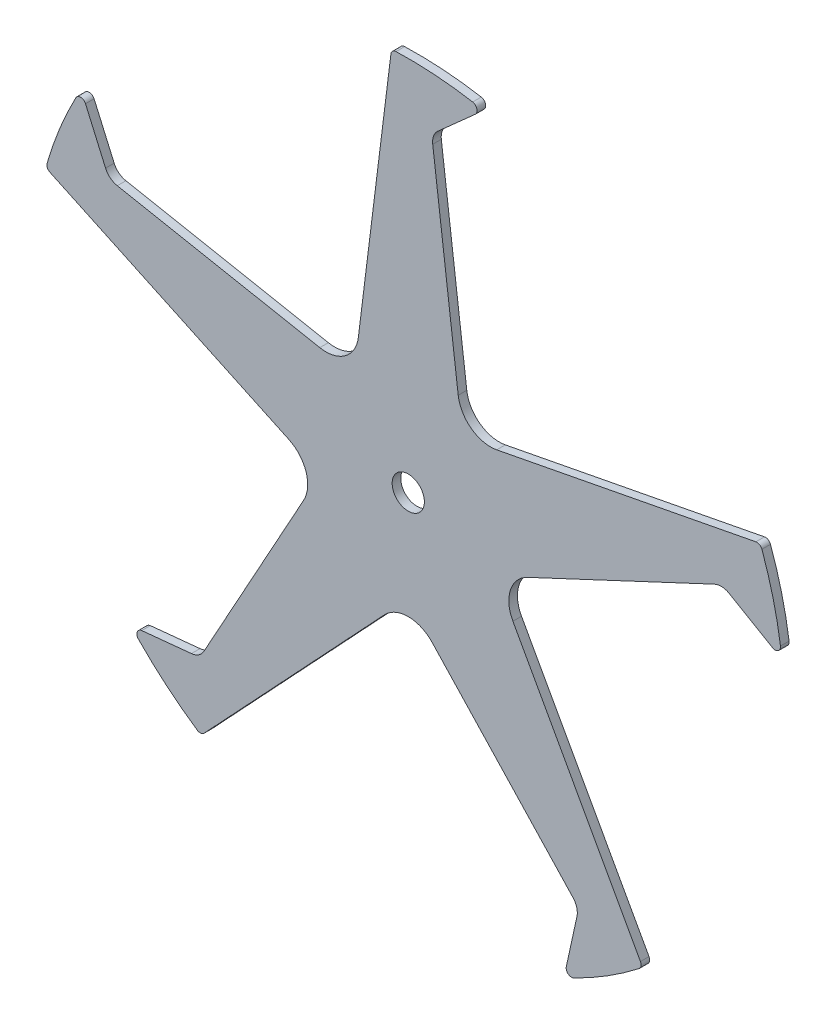
SolidWorks part; units mm, degrees
ref_plane "Front Plane" through (0, 0, 0) normal (0, 0, 1) x (1, 0, 0)
ref_plane "Top Plane" through (0, 0, 0) normal (0, 1, 0) x (1, 0, 0)
ref_plane "Right Plane" through (0, 0, 0) normal (1, 0, 0) x (0, 0, -1)
sketch "Sketch1" plane through (0, 0, 0) normal (0, 0, 1) x (1, 0, 0)
  line L0 (-46.4905, 101.7221) -> (-16.1451, 345.4365)
  line L1 (46.4905, 101.7221) -> (22.7757, 292.1841)
  line L2 (0, -284.2155) -> (0, 291.5871) construction
  line L3 (21.8025, 300) -> (-21.8025, 300) construction
  line L4 (82.3771, 75.649) -> (323.5405, 122.1007)
  line L5 (111.1098, -12.7813) -> (284.9216, 68.6289)
  line L6 (298.854, 67.9948) -> (339.0018, 44.5257)
  line L7 (292.0543, 71.9697) -> (278.5796, 113.4405) construction
  line L8 (97.4024, -54.9684) -> (216.1041, -269.9741)
  line L9 (22.1791, -109.6213) -> (153.3156, -249.7691)
  line L10 (157.0179, -263.2155) -> (147.1038, -308.6507)
  line L11 (158.697, -255.5203) -> (193.9742, -229.8899) construction
  line L12 (27.6841, 305.2386) -> (62.4109, 336.1691)
  line L13 (-22.1791, -109.6213) -> (-189.9808, -288.9539)
  line L14 (-97.4024, -54.9684) -> (-190.1674, -222.9947)
  line L15 (-201.8116, -230.6709) -> (-248.0867, -235.2823)
  line L16 (-193.9742, -229.8899) -> (-158.697, -255.5203) construction
  line L17 (-111.1098, -12.7813) -> (-333.5187, 91.3908)
  line L18 (-82.3771, 75.649) -> (-270.8455, 111.9508)
  line L19 (-281.7443, 120.6531) -> (-300.4298, 163.2382)
  line L20 (-278.5796, 113.4405) -> (-292.0543, 71.9697) construction
  arc A0 (59.9416, 344.8289) -> (-11.3455, 349.8161) centre (0, 0) ccw
  circle A1 centre (0, 0) radius 100 construction
  arc A2 (27.6841, 305.2386) -> (22.7757, 292.1841) centre (37.6608, 294.0374) ccw
  circle A3 centre (0, 0) radius 350 construction
  arc A4 (59.9416, 344.8289) -> (62.4109, 336.1691) centre (59.0853, 339.9028) cw
  arc A5 (-11.3455, 349.8161) -> (-16.1451, 345.4365) centre (-11.1834, 344.8187) ccw
  arc A6 (346.4748, 49.5501) -> (329.1889, 118.8893) centre (0, 0) ccw
  arc A7 (298.854, 67.9948) -> (284.9216, 68.6289) centre (291.284, 55.0451) ccw
  arc A8 (346.4748, 49.5501) -> (339.0018, 44.5257) centre (341.5252, 48.8423) cw
  arc A9 (329.1889, 118.8893) -> (323.5405, 122.1007) centre (324.4862, 117.1909) ccw
  arc A10 (154.1916, -314.2053) -> (214.7954, -276.3384) centre (0, 0) ccw
  arc A11 (157.0179, -263.2155) -> (153.3156, -249.7691) centre (142.3627, -260.0177) ccw
  arc A12 (154.1916, -314.2053) -> (147.1038, -308.6507) centre (151.9888, -309.7166) cw
  arc A13 (214.7954, -276.3384) -> (216.1041, -269.9741) centre (211.7269, -272.3907) ccw
  arc A14 (-251.1792, -243.7397) -> (-196.438, -289.6759) centre (0, 0) ccw
  arc A15 (-201.8116, -230.6709) -> (-190.1674, -222.9947) centre (-203.2991, -215.7448) ccw
  arc A16 (-251.1792, -243.7397) -> (-248.0867, -235.2823) centre (-247.5909, -240.2577) cw
  arc A17 (-196.438, -289.6759) -> (-189.9808, -288.9539) centre (-193.6318, -285.5376) ccw
  arc A18 (-309.4288, 163.5659) -> (-336.2008, 97.3089) centre (0, 0) ccw
  arc A19 (-281.7443, 120.6531) -> (-270.8455, 111.9508) centre (-268.0084, 126.6801) ccw
  arc A20 (-309.4288, 163.5659) -> (-300.4298, 163.2382) centre (-305.0084, 161.2292) cw
  arc A21 (-336.2008, 97.3089) -> (-333.5187, 91.3908) centre (-331.3979, 95.9188) ccw
  arc A22 (82.3771, 75.649) -> (46.4905, 101.7221) centre (76.6321, 105.4751) cw
  arc A23 (97.4024, -54.9684) -> (111.1098, -12.7813) centre (123.9934, -40.2879) cw
  arc A24 (-22.1791, -109.6213) -> (22.1791, -109.6213) centre (0, -130.3744) cw
  arc A25 (-111.1098, -12.7813) -> (-97.4024, -54.9684) centre (-123.9934, -40.2879) cw
  arc A26 (-46.4905, 101.7221) -> (-82.3771, 75.649) centre (-76.6321, 105.4751) cw
  circle A27 centre (0, 0) radius 15
  point P16 (70, 342.9286)
  point P19 (-15.6203, 349.6513)
  point P39 (50.5014, 69.5092)
  point P69 (0, -85.9181)
  point P84 (-50.5014, 69.5092)
  dimension "D2" = 700
  dimension "D3" = 200
  dimension "D5" = 70
  dimension "D6" = 30.3744
  dimension "D8" = 5
  dimension "D9" = 30
  dimension "D1" = 50
  dimension "D4" = 43.605
extrude "Linear austragen1" add sketch "Sketch1" along normal blind 8
